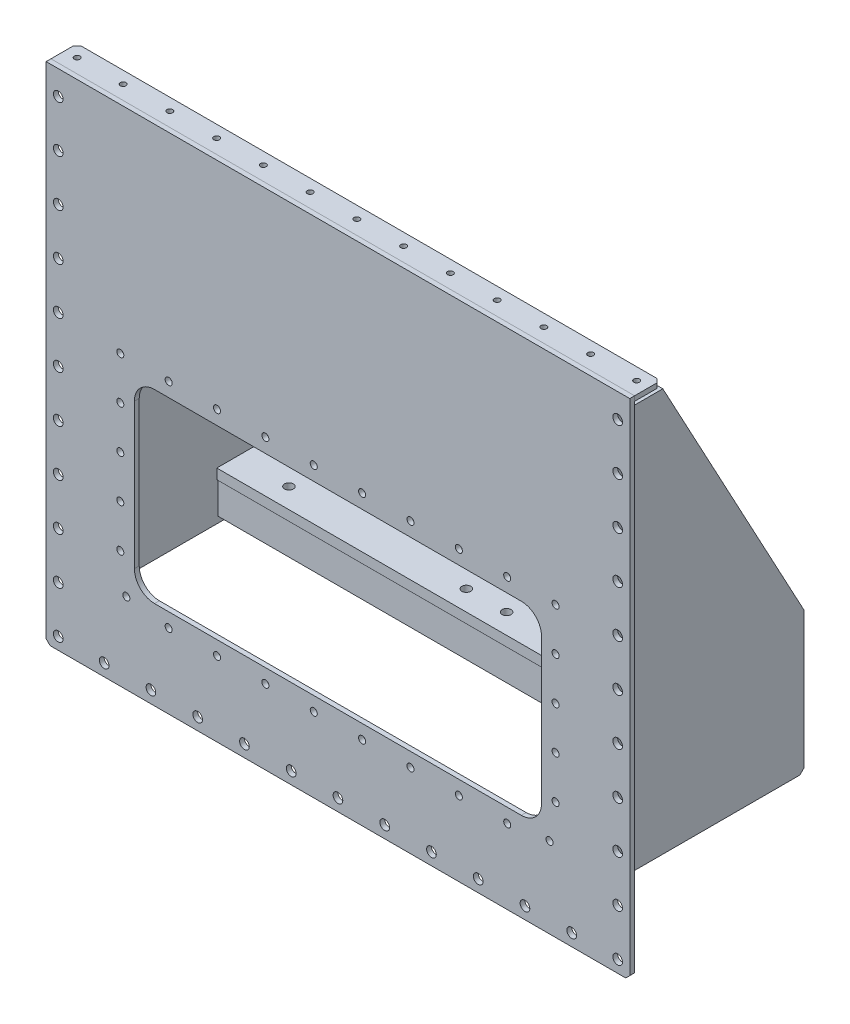
SolidWorks part; units mm, degrees
material "Q355B"
ref_plane "Front" through (0, 0, 0) normal (0, 0, 1) x (1, 0, 0)
ref_plane "Top" through (0, 0, 0) normal (0, 1, 0) x (1, 0, 0)
ref_plane "Right" through (0, 0, 0) normal (1, 0, 0) x (0, 0, -1)
sketch "Sketch1" plane through (0, 0, 0) normal (0, 0, 1) x (1, 0, 0)
  line L1 (-78.0409, 1160.7212) -> (1369.9591, 1160.7212)
  line L2 (-78.0409, 1160.7212) -> (-78.0409, -89.2788)
  line L3 (-78.0409, -89.2788) -> (1369.9591, -89.2788)
  line L4 (1369.9591, 1160.7212) -> (1369.9591, -89.2788)
extrude "Boss-Extrude1" add sketch "Sketch1" along normal blind 12
sketch "Sketch2" plane through (0, 0, 0) normal (0, 0, -1) x (-1, 0, 0)
  line L0 (-645.9591, 1160.7212) -> (-645.9591, -89.2788) construction
  line L1 (-1369.9591, 1160.7212) -> (78.0409, 1160.7212) construction
  line L2 (78.0409, -89.2788) -> (-1369.9591, -89.2788) construction
  line L3 (-1099.8021, 360.7212) -> (-71.6267, 360.7212) construction
  line L6 (-1150.9591, 590.7212) -> (-140.9591, 590.7212)
  line L7 (-1150.9591, 590.7212) -> (-1150.9591, 130.7212)
  line L8 (-1150.9591, 130.7212) -> (-140.9591, 130.7212)
  line L9 (-140.9591, 590.7212) -> (-140.9591, 130.7212)
  dimension "D1" = 800
  dimension "D2" = 460
  dimension "D3" = 1010
extrude "Cut-Extrude1" cut sketch "Sketch2" against normal blind 12
fillet "Fillet1" radius 50 4 edges at (140.9591, 590.7212, 6) (140.9591, 130.7212, 6) (1150.9591, 130.7212, 6) (1150.9591, 590.7212, 6)
chamfer "Chamfer1" distance 10 angle 45 2 edges at (-78.0409, -89.2788, 6) (1369.9591, -89.2788, 6)
sketch "Sketch3" plane through (0, 0, 0) normal (0, 0, -1) x (-1, 0, 0)
  line L0 (78.0409, 1160.7212) -> (78.0409, -79.2788) construction
  line L1 (-1369.9591, 1160.7212) -> (78.0409, 1160.7212)
  line L2 (-1369.9591, 1160.7212) -> (-1369.9591, 1148.7212)
  line L3 (-1369.9591, 1148.7212) -> (78.0409, 1148.7212)
  line L4 (78.0409, 1160.7212) -> (78.0409, 1148.7212)
extrude "Boss-Extrude2" add sketch "Sketch3" along normal blind 65 separate body
sketch "Sketch4" plane through (0, 0, 0) normal (0, 0, -1) x (-1, 0, 0)
  line L0 (78.0409, 1160.7212) -> (-1369.9591, 1160.7212) construction
  line L1 (-1369.9591, -79.2788) -> (-1369.9591, 1160.7212) construction
  line L2 (68.0409, -89.2788) -> (-1359.9591, -89.2788) construction
  line L3 (-645.9591, 1160.7212) -> (-645.9591, -89.2788) construction
  circle A0 centre (-1339.9591, 1100.7212) radius 12
  circle A1 centre (-1339.9591, 984.7212) radius 12
  circle A2 centre (-1339.9591, 868.7212) radius 12
  circle A3 centre (-1339.9591, 752.7212) radius 12
  circle A4 centre (-1339.9591, 636.7212) radius 12
  circle A5 centre (-1339.9591, 520.7212) radius 12
  circle A6 centre (-1339.9591, 404.7212) radius 12
  circle A7 centre (-1339.9591, 288.7212) radius 12
  circle A8 centre (-1339.9591, 172.7212) radius 12
  circle A9 centre (-1339.9591, 56.7212) radius 12
  circle A10 centre (-1339.9591, -59.2788) radius 12
  circle A11 centre (48.0409, -59.2788) radius 12
  circle A12 centre (48.0409, 56.7212) radius 12
  circle A13 centre (48.0409, 172.7212) radius 12
  circle A14 centre (48.0409, 288.7212) radius 12
  circle A15 centre (48.0409, 404.7212) radius 12
  circle A16 centre (48.0409, 520.7212) radius 12
  circle A17 centre (48.0409, 636.7212) radius 12
  circle A18 centre (48.0409, 752.7212) radius 12
  circle A19 centre (48.0409, 868.7212) radius 12
  circle A20 centre (48.0409, 984.7212) radius 12
  circle A21 centre (48.0409, 1100.7212) radius 12
  circle A22 centre (-1225.9591, -59.2788) radius 12
  circle A23 centre (-1109.9591, -59.2788) radius 12
  circle A24 centre (-993.9591, -59.2788) radius 12
  circle A25 centre (-877.9591, -59.2788) radius 12
  circle A26 centre (-761.9591, -59.2788) radius 12
  circle A27 centre (-645.9591, -59.2788) radius 12
  circle A28 centre (-529.9591, -59.2788) radius 12
  circle A29 centre (-413.9591, -59.2788) radius 12
  circle A30 centre (-297.9591, -59.2788) radius 12
  circle A31 centre (-181.9591, -59.2788) radius 12
  circle A32 centre (-65.9591, -59.2788) radius 12
  dimension "D1" = 60
  dimension "D2" = 30
  dimension "D4" = 30
  dimension "D5" = 114
  dimension "D3" = 11
  dimension "D6" = 11
extrude "Cut-Extrude2" cut sketch "Sketch4" against normal blind 12
sketch "Sketch5" plane through (0, 0, 0) normal (0, 0, -1) x (-1, 0, 0)
  line L0 (-645.9591, 590.7212) -> (-645.9591, 130.7212) construction
  line L1 (-1185.9591, 625.7212) -> (-105.9591, 625.7212) construction
  line L2 (-1185.9591, 625.7212) -> (-1185.9591, 95.7212) construction
  line L3 (-1185.9591, 95.7212) -> (-105.9591, 95.7212) construction
  line L4 (-105.9591, 625.7212) -> (-105.9591, 95.7212) construction
  line L5 (-190.9591, 590.7212) -> (-1100.9591, 590.7212) construction
  line L6 (-1100.9591, 130.7212) -> (-190.9591, 130.7212) construction
  line L7 (-1150.9591, 360.7212) -> (-140.9591, 360.7212) construction
  line L8 (-1150.9591, 540.7212) -> (-1150.9591, 180.7212) construction
  line L9 (-140.9591, 180.7212) -> (-140.9591, 540.7212) construction
  circle A0 centre (-1185.9591, 625.7212) radius 10
  dimension "D1" = 1080
  dimension "D2" = 530
  dimension "D3" = 265
  dimension "D4" = 540
hole_wizard "M20 Tapped Hole1" positions "Sketch7" profile "Sketch6" tap size "M20" standard "GB"
sketch "Sketch7" plane through (0, 0, 0) normal (0, 0, -1) x (-1, 0, 0)
  point P0 (-1185.9591, 625.7212)
sketch "Sketch6" plane through (1185.9591, 625.7212, 0) normal (1, 0, 0) x (0, 1, 0)
  line L0 (0, 0) -> (0, 57.7575)
  line L1 (0, 57.7575) -> (8.75, 52.5)
  line L2 (8.75, 52.5) -> (8.75, 0)
  line L5 (8.75, 0) -> (0, 0)
  line L10 (0, 57.7575) -> (-8.75, 52.5) construction
  line L11 (0, -6.35) -> (0, 107.95) construction
  dimension "螺纹孔钻头直径" = 17.5
  dimension "螺纹孔钻头深度" = 52.5
  dimension "导头角度" = 118
cosmetic thread "Cosmetic Thread1" parameters "D1"=12, "D2"=20
pattern_linear "LPattern1" count 5 spacing 106 along (0, -1, 0) of "M20 Tapped Hole1"
ref_plane "Plane1" through (645.9591, 0, 0) normal (-1, 0, 0) x (0, 0, 1)
ref_plane "Plane2" through (0, 360.7212, 0) normal (0, -1, 0) x (-1, 0, 0)
mirror "Mirror1" about plane through (645.9591, 0, 0) normal (-1, 0, 0) of "LPattern1", "M20 Tapped Hole1"
sketch "Sketch10" plane through (0, 0, 0) normal (0, 0, -1) x (-1, 0, 0)
  line L0 (-1369.9591, 1148.7212) -> (78.0409, 1148.7212) construction
  line L1 (-828.9591, 1148.7212) -> (-816.9591, 1148.7212)
  line L2 (-828.9591, 1148.7212) -> (-828.9591, 668.7212)
  line L3 (-828.9591, 668.7212) -> (-816.9591, 668.7212)
  line L4 (-816.9591, 1148.7212) -> (-816.9591, 668.7212)
  line L5 (-645.9591, 1148.7212) -> (-645.9591, 805.6959) construction
  dimension "D1" = 171
extrude "Boss-Extrude3" add sketch "Sketch10" along normal blind 50 separate body
chamfer "Chamfer2" distance 30 angle 45 1 edges at (822.9591, 668.7212, -50)
pattern_linear "LPattern5" count 2 spacing 342 along (1, 0, 0) of bodies 111
mirror "Mirror3" about plane through (645.9591, 0, 0) normal (-1, 0, 0) of bodies 112 111
chamfer "Chamfer3" distance 10 angle 45 2 edges at (-78.0409, 1154.7212, -65) (1369.9591, 1154.7212, -65)
sketch "Sketch11" plane through (0, 0, 0) normal (0, 0, -1) x (-1, 0, 0)
  line L0 (-645.9591, 130.7212) -> (-645.9591, -155.6804) construction
  line L1 (-1100.9591, 130.7212) -> (-190.9591, 130.7212) construction
  line L2 (68.0409, -89.2788) -> (-1359.9591, -89.2788) construction
  line L3 (-828.9591, -89.2788) -> (-816.9591, -89.2788)
  line L4 (-828.9591, -89.2788) -> (-828.9591, 52.7212)
  line L5 (-828.9591, 52.7212) -> (-816.9591, 52.7212)
  line L6 (-816.9591, -89.2788) -> (-816.9591, 52.7212)
  dimension "D1" = 12
  dimension "D2" = 171
extrude "Boss-Extrude4" add sketch "Sketch11" along normal blind 50 separate body
chamfer "Chamfer4" distance 30 angle 45 1 edges at (822.9591, 52.7212, -50)
pattern_linear "LPattern6" count 2 spacing 342 along (1, 0, 0) of bodies 115
mirror "Mirror4" about plane through (645.9591, 0, 0) normal (-1, 0, 0) of bodies 116 115
sketch "Sketch12" plane through (0, 1160.7212, 0) normal (0, 1, 0) x (1, 0, 0)
  line L0 (-68.0409, 65) -> (1359.9591, 65) construction
  line L1 (1369.9591, 55) -> (1369.9591, 0) construction
  circle A0 centre (1339.9591, 35) radius 7
  dimension "D1" = 30
  dimension "D2" = 30
extrude "Cut-Extrude3" cut sketch "Sketch12" against normal blind 12
sketch "Sketch13" plane through (0, 1160.7212, 0) normal (0, 1, 0) x (1, 0, 0)
  line L0 (-68.0409, 65) -> (1359.9591, 65) construction
  line L1 (-78.0409, 55) -> (-78.0409, 0) construction
  circle A0 centre (-48.0409, 35) radius 7
  circle A1 centre (65.9591, 35) radius 7
  circle A2 centre (181.9591, 35) radius 7
  circle A3 centre (297.9591, 35) radius 7
  circle A4 centre (413.9591, 35) radius 7
  circle A5 centre (529.9591, 35) radius 7
  circle A6 centre (645.9591, 35) radius 7
  circle A7 centre (761.9591, 35) radius 7
  circle A8 centre (877.9591, 35) radius 7
  circle A9 centre (993.9591, 35) radius 7
  circle A10 centre (1109.9591, 35) radius 7
  circle A11 centre (1225.9591, 35) radius 7
  dimension "D1" = 30
  dimension "D3" = 2
  dimension "D2" = 30
  dimension "D4" = 11
extrude "Cut-Extrude4" cut sketch "Sketch13" against normal blind 12
sketch "Sketch14" plane through (0, 1148.7212, 0) normal (0, -1, 0) x (1, 0, 0)
  line L1 (-34.2878, -35) -> (-41.1643, -23.0894)
  line L2 (-41.1643, -23.0894) -> (-54.9175, -23.0894)
  line L3 (-54.9175, -23.0894) -> (-61.7941, -35)
  line L4 (-61.7941, -35) -> (-54.9175, -46.9106)
  line L5 (-54.9175, -46.9106) -> (-41.1643, -46.9106)
  line L6 (-41.1643, -46.9106) -> (-34.2878, -35)
  circle A0 centre (-48.0409, -35) radius 7
  circle A1 centre (-48.0409, -35) radius 11.9106 construction
extrude "Boss-Extrude5" add sketch "Sketch14" along normal blind 12 separate body
pattern_linear "LPattern7" count 2 spacing 114 along (1, 0, 0) of "Boss-Extrude5"
pattern_linear "LPattern8" count 11 spacing 116 along (1, 0, 0) of "LPattern7"
pattern_linear "LPattern10" count 2 spacing 114 along (1, 0, 0) of bodies 132
pattern_linear "LPattern11" count 9 spacing 120 along (-1, 0, 0) of "M20 Tapped Hole1"
sketch "Sketch15" plane through (0, 0, 0) normal (0, 0, -1) x (-1, 0, 0)
  line L0 (-1185.9591, 625.7212) -> (-1185.9591, 95.7212) construction
  line L1 (-1185.9591, 95.7212) -> (-105.9591, 95.7212) construction
  circle A0 centre (-1170.9591, 110.7212) radius 7.7201
  dimension "D1" = 15
  dimension "D2" = 15
hole_wizard "M20 Tapped Hole2" positions "Sketch17" profile "Sketch16" tap size "M20" standard "GB"
sketch "Sketch17" plane through (0, 0, 0) normal (0, 0, -1) x (-1, 0, 0)
  point P0 (-1170.9591, 110.7212)
sketch "Sketch16" plane through (1170.9591, 110.7212, 0) normal (1, 0, 0) x (0, 1, 0)
  line L0 (0, 0) -> (0, 57.7575)
  line L1 (0, 57.7575) -> (8.75, 52.5)
  line L2 (8.75, 52.5) -> (8.75, 0)
  line L5 (8.75, 0) -> (0, 0)
  line L10 (0, 57.7575) -> (-8.75, 52.5) construction
  line L11 (0, -6.35) -> (0, 107.95) construction
  dimension "螺纹孔钻头直径" = 17.5
  dimension "螺纹孔钻头深度" = 52.5
  dimension "导头角度" = 118
cosmetic thread "Cosmetic Thread2" parameters "D1"=12, "D2"=20
mirror "Mirror5" about plane through (645.9591, 0, 0) normal (-1, 0, 0) of "M20 Tapped Hole2"
sketch "Sketch18" plane through (0, 0, 0) normal (0, 0, -1) x (-1, 0, 0)
  line L0 (-1185.9591, 95.7212) -> (-105.9591, 95.7212) construction
  circle A0 centre (-1065.9591, 95.7212) radius 5
  dimension "D1" = 120
hole_wizard "M20 Tapped Hole3" positions "Sketch21" profile "Sketch19" tap size "M20" standard "GB"
sketch "Sketch21" plane through (0, 0, 0) normal (0, 0, -1) x (-1, 0, 0)
  point P0 (-1065.9591, 95.7212)
sketch "Sketch19" plane through (1065.9591, 95.7212, 0) normal (1, 0, 0) x (0, 1, 0)
  line L0 (0, 0) -> (0, 57.7575)
  line L1 (0, 57.7575) -> (8.75, 52.5)
  line L2 (8.75, 52.5) -> (8.75, 0)
  line L5 (8.75, 0) -> (0, 0)
  line L10 (0, 57.7575) -> (-8.75, 52.5) construction
  line L11 (0, -6.35) -> (0, 107.95) construction
  dimension "螺纹孔钻头直径" = 17.5
  dimension "螺纹孔钻头深度" = 52.5
  dimension "导头角度" = 118
cosmetic thread "Cosmetic Thread3" parameters "D1"=12, "D2"=20
pattern_linear "LPattern12" count 8 spacing 120 along (-1, 0, 0) of "M20 Tapped Hole3"
sketch "Sketch22" plane through (0, 0, 0) normal (0, 0, -1) x (-1, 0, 0)
  line L0 (-1369.9591, -79.2788) -> (-1369.9591, 1160.7212) construction
  line L1 (-1289.9591, 1060.7212) -> (-1264.9591, 1060.7212)
  line L2 (-1289.9591, 1060.7212) -> (-1289.9591, 60.7212)
  line L3 (-1289.9591, 60.7212) -> (-1264.9591, 60.7212)
  line L4 (-1264.9591, 1060.7212) -> (-1264.9591, 60.7212)
  line L5 (68.0409, -89.2788) -> (-1359.9591, -89.2788) construction
  dimension "D1" = 25
  dimension "D2" = 80
  dimension "D3" = 1000
  dimension "D4" = 150
extrude "Boss-Extrude6" add sketch "Sketch22" along normal blind 500
sketch "Sketch23" plane through (1289.9591, 0, 0) normal (1, 0, 0) x (0, 0, -1)
  line L0 (150, 1060.7212) -> (500, 410.7212)
  line L1 (500, 1060.7212) -> (0, 1060.7212) construction
  line L2 (500, 1060.7212) -> (500, 60.7212) construction
  line L3 (150, 1060.7212) -> (500, 1060.7212)
  line L4 (500, 1060.7212) -> (500, 410.7212)
  dimension "D1" = 350
  dimension "D2" = 650
extrude "Cut-Extrude5" cut sketch "Sketch23" against normal blind 25
chamfer "Chamfer5" distance 10 angle 45 1 edges at (1277.4591, 60.7212, -500)
mirror "Mirror6" about plane through (645.9591, 0, 0) normal (-1, 0, 0) of "Chamfer5", "Cut-Extrude5", "Boss-Extrude6"
ref_plane "Plane4" through (0, 180.7212, 0) normal (0, -1, 0) x (-1, 0, 0)
sketch "Sketch27" plane through (-4.624, 180.7212, 0) normal (0, -1, 0) x (1, 0, 0)
  line L1 (28.6743, -306.5) -> (1269.5831, -306.5)
  line L2 (28.6743, -306.5) -> (28.6743, -486.5)
  line L3 (28.6743, -486.5) -> (1269.5831, -486.5)
  line L4 (1269.5831, -306.5) -> (1269.5831, -486.5)
  line L5 (1269.5831, -490) -> (1269.5831, 0) construction
  line L6 (620.5831, -456.5) -> (140.5831, -456.5) construction
  dimension "D1" = 180
  dimension "D2" = 30
extrude "Boss-Extrude7" add sketch "Sketch27" along normal blind 25 separate body contours L1 L4 L3 L2
sketch "Sketch28" plane through (0, 155.7212, 0) normal (0, -1, 0) x (1, 0, 0)
  line L1 (26.9591, -309.5) -> (1264.9591, -309.5)
  line L2 (26.9591, -309.5) -> (26.9591, -329.5)
  line L3 (26.9591, -329.5) -> (1264.9591, -329.5)
  line L4 (1264.9591, -309.5) -> (1264.9591, -329.5)
  dimension "D1" = 20
extrude "Boss-Extrude8" add sketch "Sketch28" along normal blind 80 separate body
sketch "Sketch29" plane through (0, 155.7212, 0) normal (0, -1, 0) x (1, 0, 0)
  line L0 (1264.9591, -500) -> (1264.9591, -490) construction
  line L1 (1264.9591, -495) -> (26.9591, -495)
  line L2 (1264.9591, -495) -> (1264.9591, -475)
  line L3 (1264.9591, -475) -> (26.9591, -475)
  line L4 (26.9591, -495) -> (26.9591, -475)
  line L5 (26.9591, -490) -> (26.9591, 0) construction
  dimension "D1" = 20
extrude "Boss-Extrude9" add sketch "Sketch29" along normal blind 80 separate body
sketch "Sketch30" plane through (0, 180.7212, 0) normal (0, 1, 0) x (1, 0, 0)
  line L0 (645.9591, 495) -> (645.9591, 226.5675) construction
  line L1 (26.9591, 495) -> (1264.9591, 495) construction
  line L2 (645.9591, 6.6) -> (645.9591, -6.6) construction
  point P7 (1135.9591, 436.5)
  point P9 (1135.9591, 356.5)
  point P11 (695.9591, 436.5)
  point P13 (695.9591, 356.5)
  point P23 (595.9591, 356.5)
  point P24 (595.9591, 436.5)
  point P25 (155.9591, 356.5)
  point P26 (155.9591, 436.5)
ref_plane "Plane5" through (645.9591, 0, 0) normal (-1, 0, 0) x (0, 0, 1)
hole_wizard "Ø22.0 (22) Hole2" positions "Sketch34" profile "Sketch33" hole size "Ø22.0" standard "GB" end condition up to next
sketch "Sketch34" plane through (0, 180.7212, 0) normal (0, 1, 0) x (1, 0, 0)
  point P12 (1135.9591, 356.5)
  point P15 (1135.9591, 436.5)
  point P18 (695.9591, 356.5)
  point P21 (695.9591, 436.5)
  point P29 (155.9591, 436.5)
  point P32 (595.9591, 436.5)
  point P35 (155.9591, 356.5)
  point P38 (595.9591, 356.5)
sketch "Sketch33" plane through (1135.9591, 180.7212, -356.5) normal (1, 0, 0) x (0, 0, 1)
  line L0 (0, 0) -> (0, 25.001)
  line L1 (0, 25.001) -> (11, 25.001)
  line L2 (11, 25.001) -> (11, 0)
  line L5 (11, 0) -> (0, 0)
  line L11 (0, -6.35) -> (0, 107.95) construction
  dimension "通孔孔直径" = 22
  dimension "通孔孔深度" = 25.001
equation "\"零件重量\"= IIF ( \"SW-质量\" > 100 , int ( \"SW-质量\" ) , \"SW-质量\" )"
